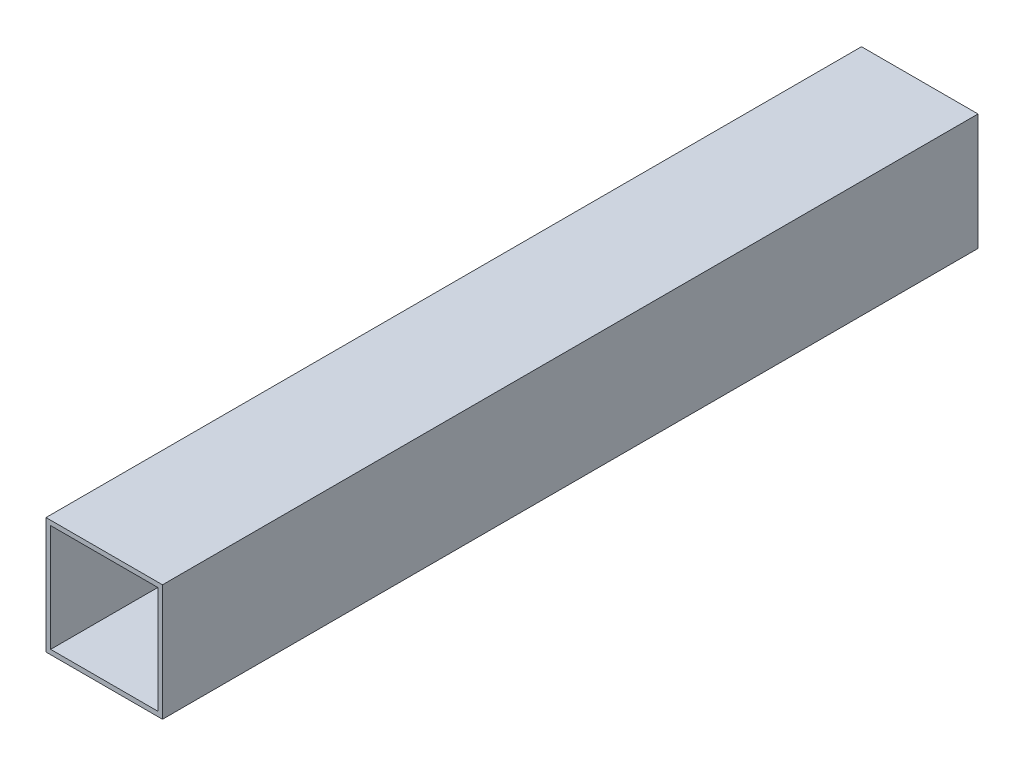
from build123d import *

# Parameters (mm, degrees)
SKETCH1_W           = 50
SKETCH1_H           = 50
SKETCH1_W_2         = 46
SKETCH1_H_2         = 46
BOSS_EXTRUDE1_DEPTH = 350


with BuildPart() as part:
    # Sketch1 → Boss-Extrude1 (new body)
    with BuildSketch(Plane.XY):
        Rectangle(SKETCH1_W, SKETCH1_H)
        Rectangle(SKETCH1_W_2, SKETCH1_H_2, mode=Mode.SUBTRACT)
    extrude(amount=BOSS_EXTRUDE1_DEPTH)


solid = part.part
